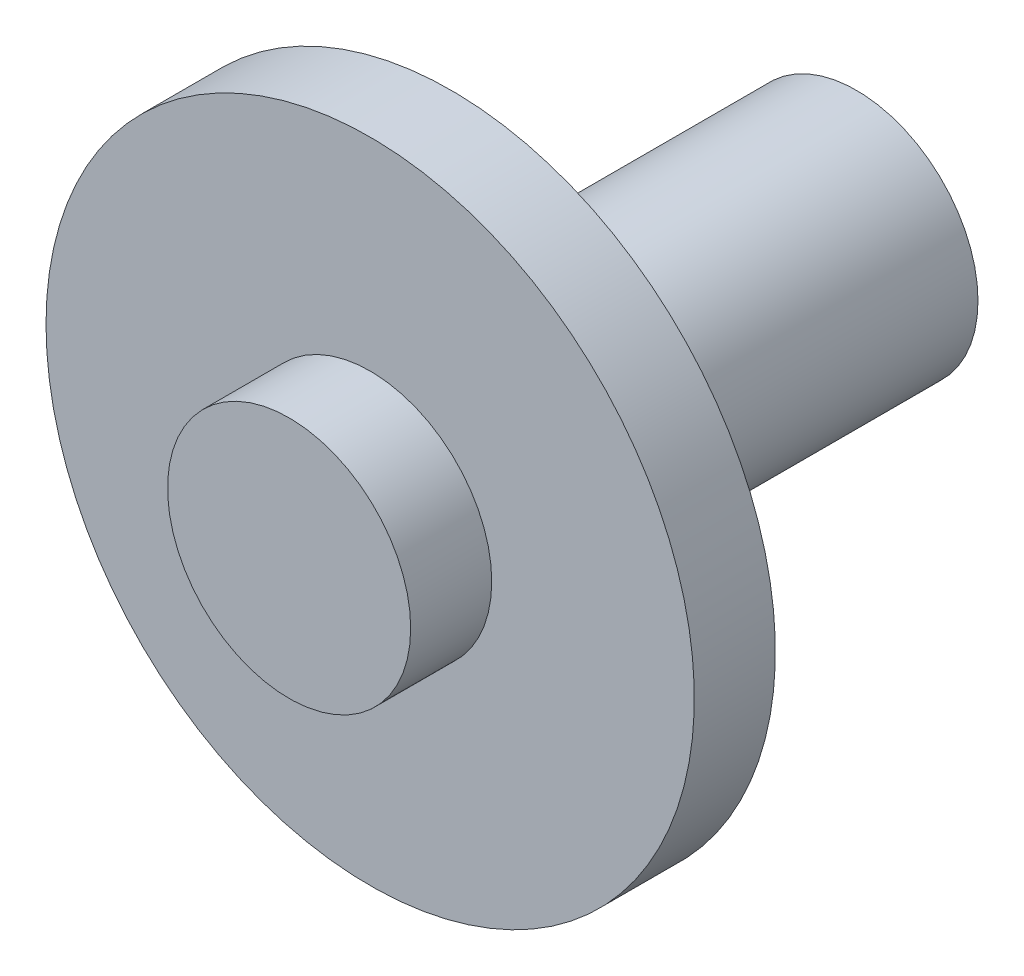
from build123d import *

# Parameters (mm, degrees)
SKETCH_1_R           = 1.5
BOSS_EXTRUDE_1_DEPTH = 1
SKETCH_2_R           = 4
BOSS_EXTRUDE_2_DEPTH = 1
SKETCH_3_R           = 2.5
BOSS_EXTRUDE_3_DEPTH = 1
BOSS_EXTRUDE_START   = 4
SKETCH_4_R           = 1.5
BOSS_EXTRUDE_4_DEPTH = 4


with BuildPart() as part:
    # Sketch 1 → Boss-Extrude 1 (new body)
    with BuildSketch(Plane.XY):
        Circle(SKETCH_1_R)
    extrude(amount=BOSS_EXTRUDE_1_DEPTH)

    # Sketch 2 → Boss-Extrude 2 (add)
    with BuildSketch(Plane(origin=(0, 0, 0), x_dir=(-1, 0, 0), z_dir=(0, 0, -1))):
        Circle(SKETCH_2_R)
    extrude(amount=BOSS_EXTRUDE_2_DEPTH)

    # Sketch 3 → Boss-Extrude 3 (add)
    with BuildSketch(Plane(origin=(0, 0, -1), x_dir=(-1, 0, 0), z_dir=(0, 0, -1))):
        Circle(SKETCH_3_R)
    extrude(amount=BOSS_EXTRUDE_3_DEPTH)

    # Sketch 4 → Boss-Extrude 4 (add)
    with BuildSketch(Plane(origin=(0, 0, -2), x_dir=(-1, 0, 0), z_dir=(0, 0, -1)).offset(BOSS_EXTRUDE_START)):
        with Locations(Location((0, 0, 0), (0, 0, 180))):
            Circle(SKETCH_4_R)
    extrude(amount=-BOSS_EXTRUDE_4_DEPTH)

    # Sketch 5 → Cut-Revolve 2 (revolve, cut)
    with BuildSketch(Plane(origin=(0, 0, 0), x_dir=(1, 0, 0), z_dir=(0, 1, 0))):
        with BuildLine():
            Line((1.5, 2.003149648), (2.5, 2.000004945))
            Line((2.5, 2.000004945), (2.5, 1))
            ThreePointArc((2.5, 1), (1.791778774, 1.294007363), (1.5, 2.003149648))
        make_face()
    revolve(axis=Axis((0, 0, -2.003149648), (0, 0, -1)), mode=Mode.SUBTRACT)


solid = part.part
